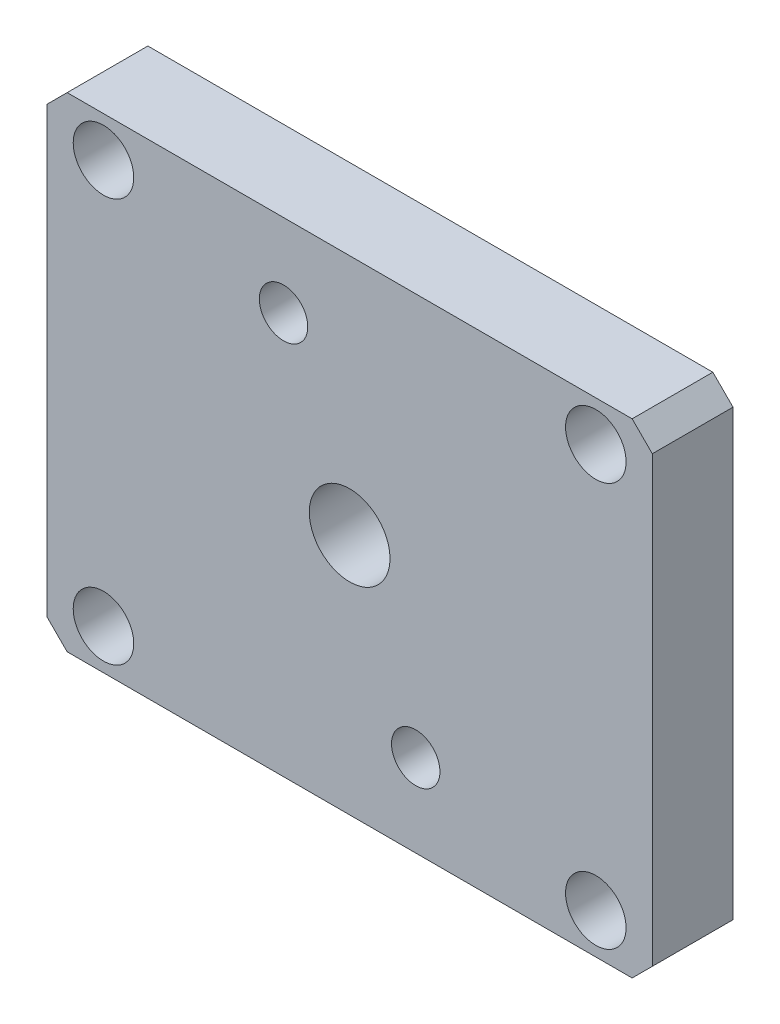
from build123d import *

# Parameters (mm, degrees)
BOSS_EXTRUDE1_DEPTH     = 20
CUT_EXTRUDE1_DEPTH      = 99.107084352
CUT_EXTRUDE1_DEPTH_BACK = 99.107084352
SKETCH3_R               = 7.5
SKETCH4_R               = 10
CUT_EXTRUDE2_DEPTH      = 59
CUT_EXTRUDE3_REACH      = 100.107
SKETCH5_R               = 6


with BuildPart() as part:
    # Sketch2 → Boss-Extrude1 (new body)
    with BuildSketch(Plane.XY):
        Polygon((75, -55), (70, -60), (-70, -60), (-75, -55), (-75, 55), (-70, 60), (70, 60), (75, 55), align=None)
    extrude(amount=BOSS_EXTRUDE1_DEPTH)

    # Sketch3 → Cut-Extrude1 (cut, two sides: drawn at the far end of the back side and taken through both)
    with BuildSketch(Plane(origin=(0, 0, 0), x_dir=(-1, 0, 0), z_dir=(0, 0, -1)).offset(-CUT_EXTRUDE1_DEPTH_BACK)):
        with Locations((61, -50)):
            Circle(SKETCH3_R)
        with Locations((61, 50)):
            Circle(SKETCH3_R)
        with Locations((-61, -50)):
            Circle(SKETCH3_R)
        with Locations((-61, 50)):
            Circle(SKETCH3_R)
    extrude(amount=CUT_EXTRUDE1_DEPTH + CUT_EXTRUDE1_DEPTH_BACK, mode=Mode.SUBTRACT)

    # Sketch4 → Cut-Extrude2 (cut)
    with BuildSketch(Plane(origin=(0, 0, 0), x_dir=(-1, 0, 0), z_dir=(0, 0, -1))):
        Circle(SKETCH4_R)
    extrude(amount=-CUT_EXTRUDE2_DEPTH, mode=Mode.SUBTRACT)

    # Sketch5 → Cut-Extrude3 (cut, up to next)
    with BuildSketch(Plane(origin=(0, 0, 0), x_dir=(-1, 0, 0), z_dir=(0, 0, -1)), mode=Mode.PRIVATE) as cut_extrude3_sk1:
        with Locations((-16.378850905, -39.542043991)):
            Circle(SKETCH5_R)
    cut_extrude3_tool1 = extrude(cut_extrude3_sk1.sketch, amount=-CUT_EXTRUDE3_REACH, mode=Mode.PRIVATE) & part.part
    # Sketch5 → Cut-Extrude3 (cut, up to next)
    with BuildSketch(Plane(origin=(0, 0, 0), x_dir=(-1, 0, 0), z_dir=(0, 0, -1)), mode=Mode.PRIVATE) as cut_extrude3_sk2:
        with Locations((16.378850905, 39.542043991)):
            Circle(SKETCH5_R)
    cut_extrude3_tool2 = extrude(cut_extrude3_sk2.sketch, amount=-CUT_EXTRUDE3_REACH, mode=Mode.PRIVATE) & part.part
    add(cut_extrude3_tool1.solids().sort_by_distance((16.378851, -39.542044, 0))[0], mode=Mode.SUBTRACT)
    add(cut_extrude3_tool2.solids().sort_by_distance((-16.378851, 39.542044, 0))[0], mode=Mode.SUBTRACT)


solid = part.part
